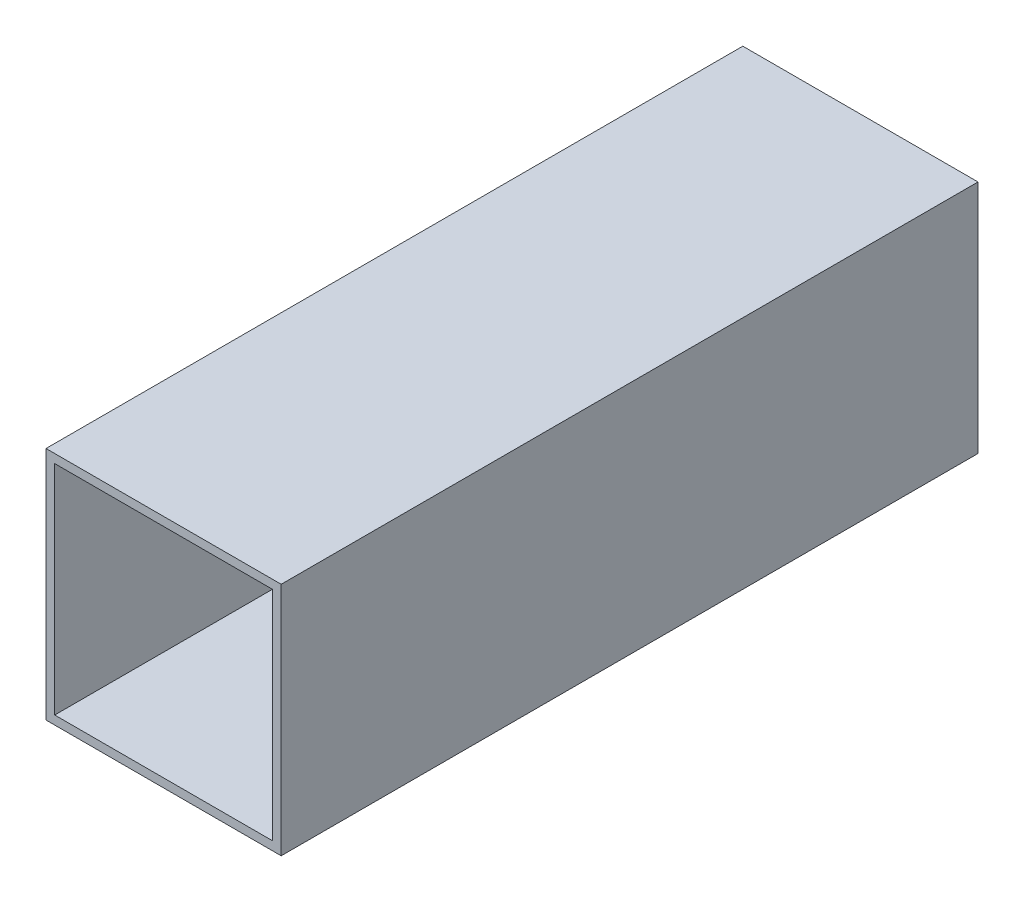
SolidWorks part; units mm, degrees
ref_plane "Front Plane" through (0, 0, 0) normal (0, 0, 1) x (1, 0, 0)
ref_plane "Top Plane" through (0, 0, 0) normal (0, 1, 0) x (1, 0, 0)
ref_plane "Right Plane" through (0, 0, 0) normal (1, 0, 0) x (0, 0, -1)
sketch "Sketch1" plane through (0, 0, 0) normal (0, 0, 1) x (1, 0, 0)
  line L1 (125, 125) -> (-125, 125)
  line L2 (125, 125) -> (125, -125)
  line L3 (125, -125) -> (-125, -125)
  line L4 (-125, 125) -> (-125, -125)
  line L5 (125, 125) -> (-125, -125) construction
  line L6 (125, -125) -> (-125, 125) construction
  point P0 (0, 0)
  dimension "D1" = 250
extrude "Extrude-Thin1" add sketch "Sketch1" along normal blind 800 thin
